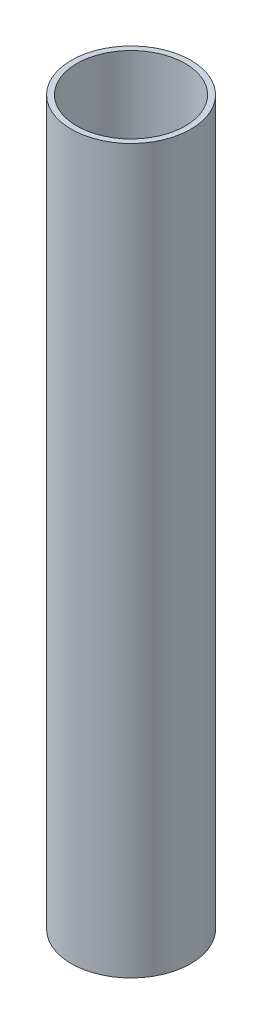
from build123d import *

# Parameters (mm, degrees)
SKETCH_1_R      = 2.15
SKETCH_1_R_2    = 1.95
EXTRUDE_1_DEPTH = 26


with BuildPart() as part:
    # 草图1 → 拉伸-薄壁1 (new body)
    with BuildSketch(Plane(origin=(0, 0, 0), x_dir=(1, 0, 0), z_dir=(0, 1, 0))):
        Circle(SKETCH_1_R)
        Circle(SKETCH_1_R_2, mode=Mode.SUBTRACT)
    extrude(amount=EXTRUDE_1_DEPTH)


solid = part.part
